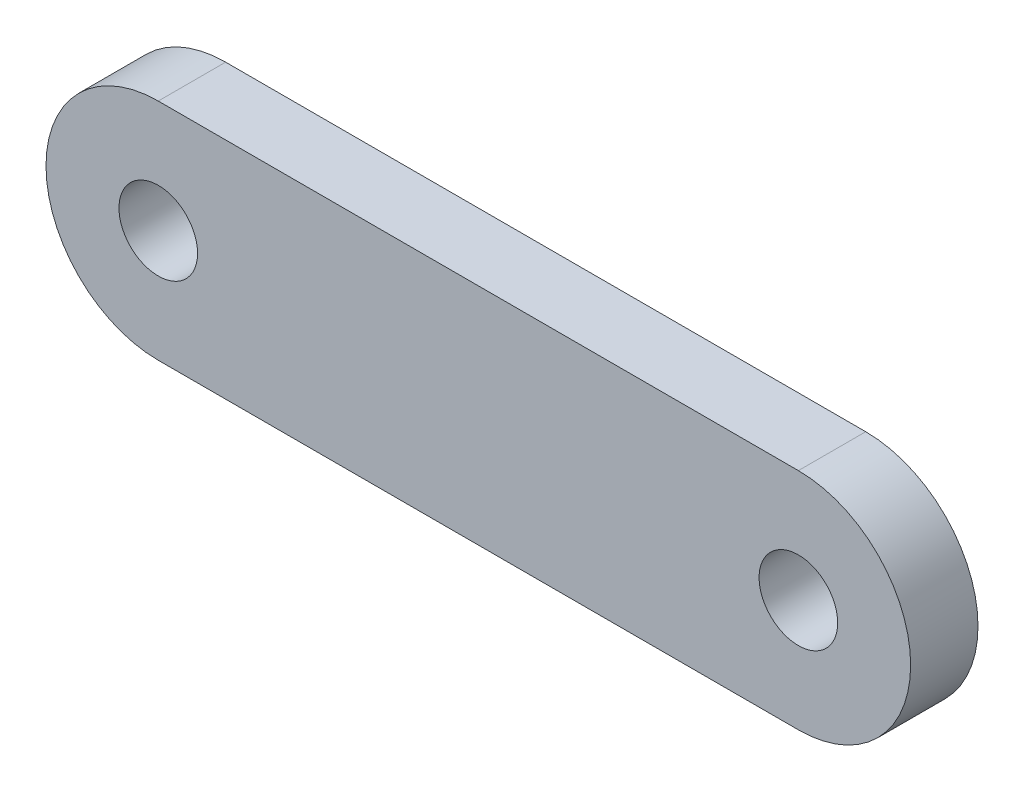
SolidWorks part; units mm, degrees
ref_plane "Front Plane" through (0, 0, 0) normal (0, 0, 1) x (1, 0, 0)
ref_plane "Top Plane" through (0, 0, 0) normal (0, 1, 0) x (1, 0, 0)
ref_plane "Right Plane" through (0, 0, 0) normal (1, 0, 0) x (0, 0, -1)
sketch "Sketch1" plane through (0, 0, 0) normal (0, 0, 1) x (1, 0, 0)
  line L0 (3.3, 0) -> (-3.3, 0) construction
  line L1 (0, 10) -> (57.02, 10)
  line L2 (0, 0) -> (158.2009, 0) construction
  line L3 (0, -10) -> (57.02, -10)
  arc A0 (0, 10) -> (0, -10) centre (0, 0) ccw
  arc A1 (57.02, -10) -> (57.02, 10) centre (57.02, 0) ccw
  dimension "D1" = 57.02
  dimension "D2" = 20
  dimension "D3" = 20
extrude "Boss-Extrude1" add sketch "Sketch1" along normal blind 6
sketch "Sketch2" plane through (0, 0, 6) normal (0, 0, 1) x (1, 0, 0)
  circle A0 centre (0, 0) radius 3.5
  circle A1 centre (57.02, 0) radius 3.5
  dimension "D1" = 7
  dimension "D2" = 7
extrude "Cut-Extrude1" cut sketch "Sketch2" against normal blind 95
